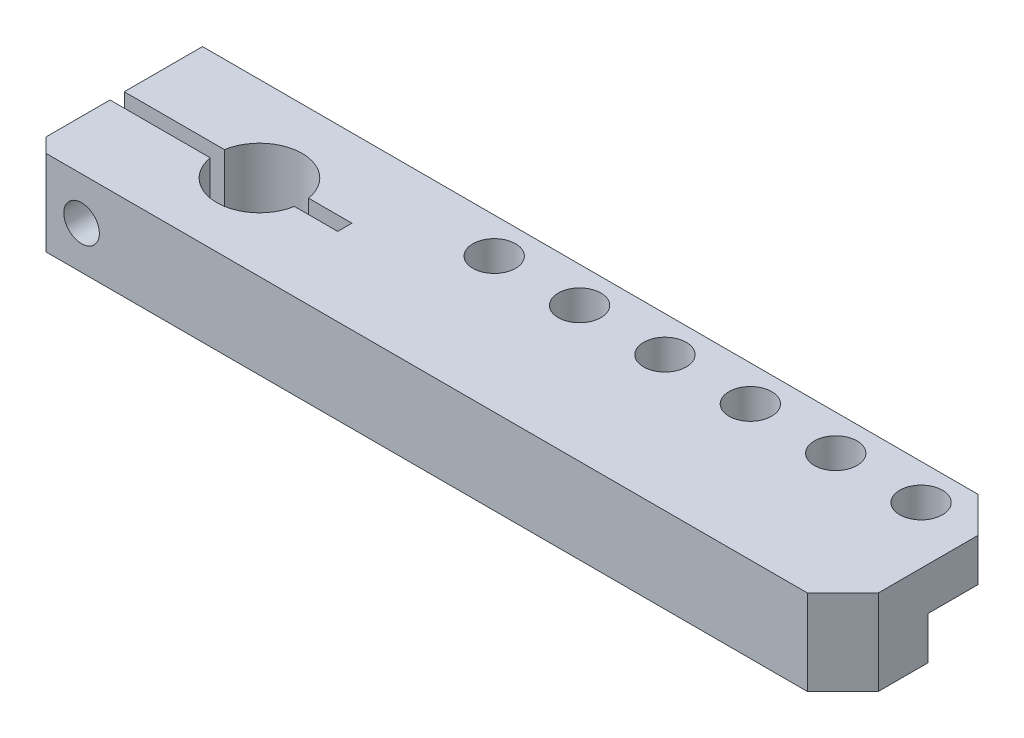
SolidWorks part; units mm, degrees
ref_plane "Front Plane" through (0, 0, 0) normal (0, 0, 1) x (1, 0, 0)
ref_plane "Top Plane" through (0, 0, 0) normal (0, 1, 0) x (1, 0, 0)
ref_plane "Right Plane" through (0, 0, 0) normal (1, 0, 0) x (0, 0, -1)
sketch "Sketch1" plane through (0, 0, 0) normal (0, 1, 0) x (1, 0, 0)
  line L0 (0, 0) -> (50000, 0) construction
  line L1 (-32.5, 6) -> (32.5, 6)
  line L2 (-32.5, 6) -> (-32.5, -6)
  line L3 (-32.5, -6) -> (32.5, -6)
  line L4 (32.5, 6) -> (32.5, -6)
  line L5 (-32.5, 6) -> (32.5, -6) construction
  line L6 (-32.5, -6) -> (32.5, 6) construction
  circle A0 centre (-22.5, 0) radius 3
  point P0 (0, 0)
  dimension "D1" = 6
  dimension "D2" = 10
  dimension "D3" = 65
  dimension "D4" = 12
extrude "Boss-Extrude1" add sketch "Sketch1" along normal blind 6
sketch "Sketch2" plane through (0, 0, 0) normal (0, -1, 0) x (1, 0, 0)
  line L0 (0, 0) -> (-50000, 0) construction
  line L1 (-32.5, -6) -> (-32.5, 6) construction
  line L3 (-48.5, 0.5) -> (-16.5, 0.5)
  line L4 (-48.5, 0.5) -> (-48.5, -0.5)
  line L5 (-48.5, -0.5) -> (-16.5, -0.5)
  line L6 (-16.5, 0.5) -> (-16.5, -0.5)
  line L7 (-48.5, 0.5) -> (-16.5, -0.5) construction
  line L8 (-48.5, -0.5) -> (-16.5, 0.5) construction
  point P5 (-32.5, 0)
  point P6 (-32.5, 0)
  dimension "D1" = 1
  dimension "D2" = 16
extrude "Cut-Extrude1" cut sketch "Sketch2" against normal through all
sketch "Sketch4" plane through (0, 0, -6) normal (0, 0, -1) x (-1, 0, 0)
  line L0 (-32.5, 6) -> (32.5, 6) construction
  line L1 (32.5, 6) -> (32.5, 0) construction
  circle A0 centre (29, 3) radius 1.75
  dimension "D1" = 3.5
  dimension "D2" = 3
  dimension "D3" = 3.5
extrude "Cut-Extrude3" cut sketch "Sketch4" against normal blind 6
hole_wizard "M3 Tapped Hole1" positions "3DSketch1" profile "Sketch5" tap size "M3" standard "Gb" end condition through all
sketch3d "3DSketch1"
  line L0 (-29, 3, -0.5) -> (-29, 3, -6) construction
  point P0 (-29, 3, 0.5)
  dimension "D1" = 0
sketch "Sketch5" plane through (-29, 3, 0.5) normal (1, 0, 0) x (0, 1, 0)
  line L0 (0, 0) -> (0, 5.5)
  line L1 (0, 5.5) -> (1.25, 5.5)
  line L2 (1.25, 5.5) -> (1.25, 0)
  line L5 (1.25, 0) -> (0, 0)
  line L11 (0, -6.35) -> (0, 107.95) construction
  dimension "通孔螺纹孔钻头直径" = 2.5
  dimension "通孔螺纹孔钻头深度" = 5.5
cosmetic thread "Hole Thread1" parameters "D2"=3
sketch "Sketch10" plane through (0, 0, 0) normal (0, -1, 0) x (1, 0, 0)
  line L1 (32.5, -6) -> (-15.5, -6)
  line L2 (32.5, -6) -> (32.5, 0)
  line L3 (32.5, 0) -> (-15.5, 0)
  line L4 (-15.5, -6) -> (-15.5, 0)
  dimension "D1" = 48
  dimension "D2" = 6
extrude "Cut-Extrude4" cut sketch "Sketch10" against normal blind 3
hole_wizard "Ø3.0 (3) Diameter Hole1" positions "3DSketch2" profile "Sketch7" hole size "Ø3.0" standard "Gb" end condition through all
sketch3d "3DSketch2"
  point P0 (20.5, 0, -3.5)
  dimension "D1" = 12
  dimension "D2" = 2.5
sketch "Sketch7" plane through (20.5, 0, -3.5) normal (1, 0, 0) x (0, 0, -1)
  line L0 (0, 0) -> (0, 6)
  line L1 (0, 6) -> (1.5, 6)
  line L2 (1.5, 6) -> (1.5, 0)
  line L5 (1.5, 0) -> (0, 0)
  line L11 (0, -6.35) -> (0, 107.95) construction
  dimension "通孔孔直径" = 3
  dimension "通孔孔深度" = 6
pattern_linear "LPattern1" count 6 spacing 6 along (-1, 0, 0) of "Ø3.0 (3) Diameter Hole1"
fillet "Fillet1" radius 3 1 edges at (-15.5, 1.5, 0)
sketch "Sketch11" plane through (0, 0, 0) normal (0, -1, 0) x (1, 0, 0)
  line L0 (-15.5, -6) -> (32.5, -6) construction
  line L1 (32.5, 6) -> (24.5, 6)
  line L2 (32.5, 6) -> (32.5, -6)
  line L3 (32.5, -6) -> (24.5, -6)
  line L4 (24.5, 6) -> (24.5, -6)
  dimension "D1" = 8
extrude "Cut-Extrude5" cut sketch "Sketch11" against normal blind 10
chamfer "Chamfer1" distance 1 angle 45 1 edges at (-32.5, 3, 6)
chamfer "Chamfer2" distance 2.5 angle 45 2 edges at (24.5, 4.5, -6) (24.5, 3, 6)
